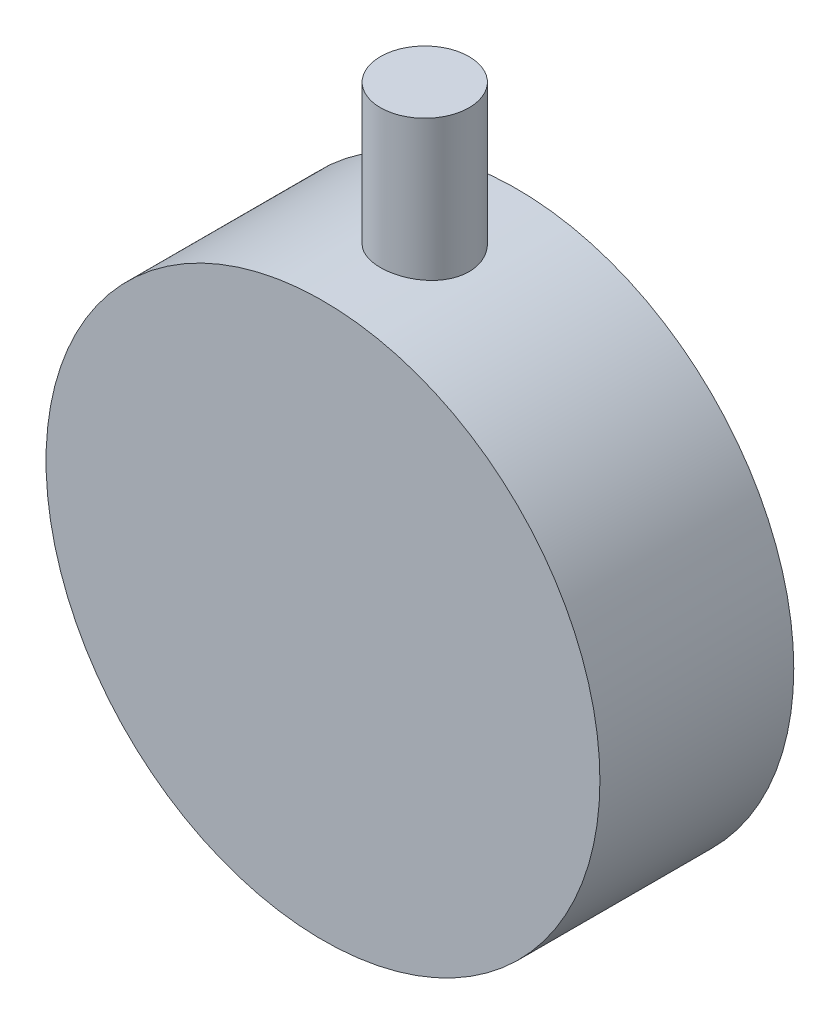
from build123d import *

# Parameters (mm, degrees)
SKETCH1_R           = 50
BOSS_EXTRUDE1_DEPTH = 35
SKETCH2_R           = 8
BOSS_EXTRUDE2_DEPTH = 75


with BuildPart() as part:
    # Sketch1 → Boss-Extrude1 (new body)
    with BuildSketch(Plane.XY):
        Circle(SKETCH1_R)
    extrude(amount=BOSS_EXTRUDE1_DEPTH)

    # Sketch2 → Boss-Extrude2 (add)
    with BuildSketch(Plane(origin=(0, 0, 0), x_dir=(1, 0, 0), z_dir=(0, 1, 0))):
        with Locations(Location((0, -16.62435188, 0), (0, 0, 90))):
            Circle(SKETCH2_R)
    extrude(amount=BOSS_EXTRUDE2_DEPTH)


solid = part.part
